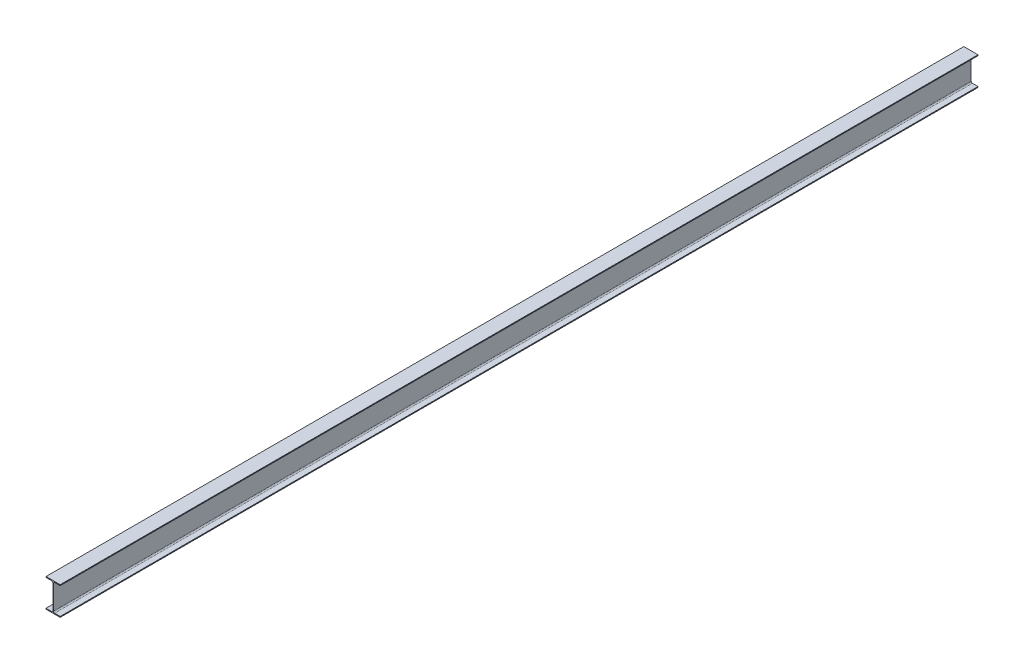
from build123d import *

# Parameters (mm, degrees)
BOSS_EXTRUDE1_DEPTH = 9710


with BuildPart() as part:
    # Sketch1 → Boss-Extrude1 (new body)
    with BuildSketch(Plane.XY):
        with BuildLine():
            Line((75, 0), (-75, 0))
            Line((-75, 0), (-75, 9))
            Line((-75, 9), (-16.25, 9))
            ThreePointArc((-16.25, 9), (-7.057611845, 12.807611845), (-3.25, 22))
            Line((-3.25, 22), (-3.25, 278))
            ThreePointArc((-3.25, 278), (-7.057611845, 287.192388155), (-16.25, 291))
            Line((-16.25, 291), (-75, 291))
            Line((-75, 291), (-75, 300))
            Line((-75, 300), (75, 300))
            Line((75, 300), (75, 291))
            Line((75, 291), (16.25, 291))
            ThreePointArc((16.25, 291), (7.057611845, 287.192388155), (3.25, 278))
            Line((3.25, 278), (3.25, 22))
            ThreePointArc((3.25, 22), (7.057611845, 12.807611845), (16.25, 9))
            Line((16.25, 9), (75, 9))
            Line((75, 9), (75, 0))
        make_face()
    extrude(amount=BOSS_EXTRUDE1_DEPTH)


solid = part.part
